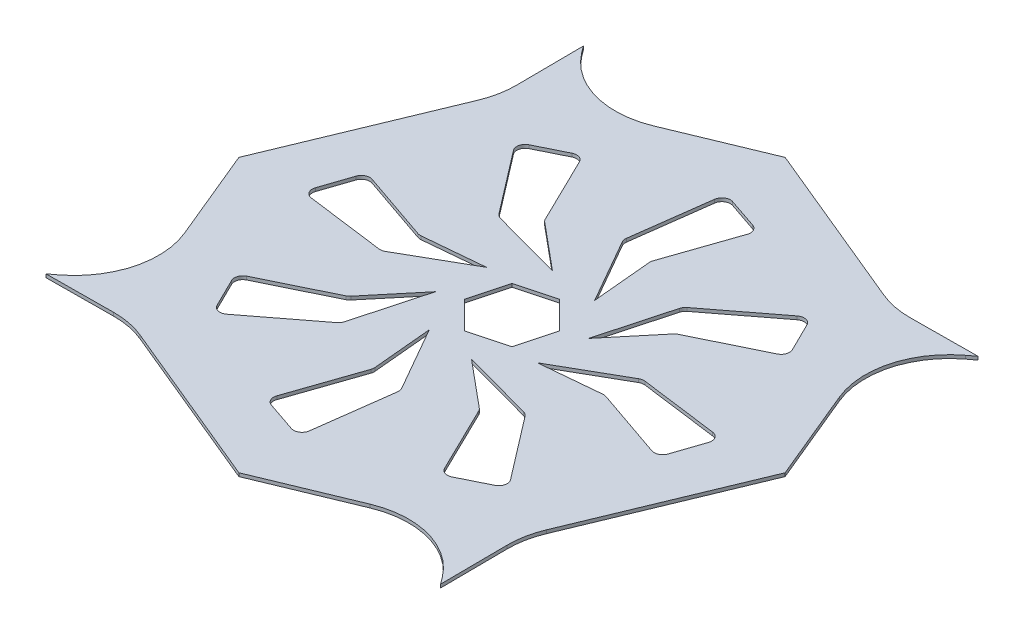
SolidWorks part; units mm, degrees
material "45"
ref_plane "Front Plane" through (0, 0, 0) normal (0, 0, 1) x (1, 0, 0)
ref_plane "Top Plane" through (0, 0, 0) normal (0, 1, 0) x (1, 0, 0)
ref_plane "Right Plane" through (0, 0, 0) normal (1, 0, 0) x (0, 0, -1)
sketch "Sketch1" plane through (0, 0, 0) normal (0, 1, 0) x (1, 0, 0)
  line L1 (114.805, -114.805) -> (162.3588, 0)
  line L2 (162.3588, 0) -> (114.805, 114.805)
  line L3 (114.805, 114.805) -> (0, 162.3588)
  line L4 (0, 162.3588) -> (-114.805, 114.805)
  line L5 (-114.805, 114.805) -> (-162.3588, 0)
  line L6 (-162.3588, 0) -> (-114.805, -114.805)
  line L7 (-114.805, -114.805) -> (0, -162.3588)
  line L8 (0, -162.3588) -> (114.805, -114.805)
  circle A0 centre (0, 0) radius 150 construction
  dimension "D1" = 300
extrude "Boss-Extrude1" add sketch "Sketch1" along normal blind 2
sketch "Sketch2" plane through (0, 2, 0) normal (0, 1, 0) x (1, 0, 0)
  line L0 (0, 0) -> (46.3685, 0) construction
  line L1 (22.3071, 5.9772) -> (5.9772, 22.3071)
  line L2 (5.9772, 22.3071) -> (-16.3299, 16.3299)
  line L3 (-16.3299, 16.3299) -> (-22.3071, -5.9772)
  line L4 (-22.3071, -5.9772) -> (-5.9772, -22.3071)
  line L5 (-5.9772, -22.3071) -> (16.3299, -16.3299)
  line L6 (16.3299, -16.3299) -> (22.3071, 5.9772)
  line L7 (0, 0) -> (16.3299, -16.3299) construction
  circle A0 centre (0, 0) radius 20 construction
  dimension "D1" = 40
  dimension "D2" = 45
extrude "Cut-Extrude1" cut sketch "Sketch2" against normal blind 10
sketch "Sketch3" plane through (0, 2, 0) normal (0, 1, 0) x (1, 0, 0)
  line L0 (7.1807, 123.975) -> (25.2073, 117.8588)
  line L1 (28.3287, 111.4971) -> (13.9987, 69.8505)
  line L2 (13.7476, 67.7664) -> (17.0204, 32.1308)
  line L3 (17.0204, 32.1308) -> (-4.8848, 70.4296)
  line L4 (-5.5015, 73.5667) -> (0.6173, 119.8948)
  line L5 (92.7411, 82.586) -> (101.163, 65.5145)
  line L6 (98.8718, 58.8089) -> (59.2903, 39.4932)
  line L7 (57.6391, 38.197) -> (34.7552, 10.6847)
  line L8 (34.7552, 10.6847) -> (46.3472, 53.2553)
  line L9 (48.1294, 55.9097) -> (85.2149, 84.3419)
  line L10 (123.975, -7.1807) -> (117.8588, -25.2073)
  line L11 (111.4971, -28.3287) -> (69.8505, -13.9987)
  line L12 (67.7664, -13.7476) -> (32.1308, -17.0204)
  line L13 (32.1308, -17.0204) -> (70.4296, 4.8848)
  line L14 (73.5667, 5.5015) -> (119.8948, -0.6173)
  line L15 (82.586, -92.7411) -> (65.5145, -101.163)
  line L16 (58.8089, -98.8718) -> (39.4932, -59.2903)
  line L17 (38.197, -57.6391) -> (10.6847, -34.7552)
  line L18 (10.6847, -34.7552) -> (53.2553, -46.3472)
  line L19 (55.9097, -48.1294) -> (84.3419, -85.2149)
  line L20 (-7.1807, -123.975) -> (-25.2073, -117.8588)
  line L21 (-28.3287, -111.4971) -> (-13.9987, -69.8505)
  line L22 (-13.7476, -67.7664) -> (-17.0204, -32.1308)
  line L23 (-17.0204, -32.1308) -> (4.8848, -70.4296)
  line L24 (5.5015, -73.5667) -> (-0.6173, -119.8948)
  line L25 (-92.7411, -82.586) -> (-101.163, -65.5145)
  line L26 (-98.8718, -58.8089) -> (-59.2903, -39.4932)
  line L27 (-57.6391, -38.197) -> (-34.7552, -10.6847)
  line L28 (-34.7552, -10.6847) -> (-46.3472, -53.2553)
  line L29 (-48.1294, -55.9097) -> (-85.2149, -84.3419)
  line L30 (-123.975, 7.1807) -> (-117.8588, 25.2073)
  line L31 (-111.4971, 28.3287) -> (-69.8505, 13.9987)
  line L32 (-67.7664, 13.7476) -> (-32.1308, 17.0204)
  line L33 (-32.1308, 17.0204) -> (-70.4296, -4.8848)
  line L34 (-73.5667, -5.5015) -> (-119.8948, 0.6173)
  line L35 (-82.586, 92.7411) -> (-65.5145, 101.163)
  line L36 (-58.8089, 98.8718) -> (-39.4932, 59.2903)
  line L37 (-38.197, 57.6391) -> (-10.6847, 34.7552)
  line L38 (-10.6847, 34.7552) -> (-53.2553, 46.3472)
  line L39 (-55.9097, 48.1294) -> (-84.3419, 85.2149)
  arc A0 (13.9987, 69.8505) -> (13.7476, 67.7664) centre (18.7267, 68.2237) ccw
  arc A1 (-4.8848, 70.4296) -> (-5.5015, 73.5667) centre (-0.5445, 72.912) cw
  arc A2 (0.6173, 119.8948) -> (7.1807, 123.975) centre (5.5743, 119.2401) cw
  arc A3 (28.3287, 111.4971) -> (25.2073, 117.8588) centre (23.6008, 113.1239) ccw
  circle A4 centre (0, 0) radius 14.7187 construction
  arc A5 (59.2903, 39.4932) -> (57.6391, 38.197) centre (61.4832, 34.9997) ccw
  arc A6 (46.3472, 53.2553) -> (48.1294, 55.9097) centre (51.1715, 51.9416) cw
  arc A7 (85.2149, 84.3419) -> (92.7411, 82.586) centre (88.2571, 80.3739) cw
  arc A8 (98.8718, 58.8089) -> (101.163, 65.5145) centre (96.679, 63.3024) ccw
  arc A9 (69.8505, -13.9987) -> (67.7664, -13.7476) centre (68.2237, -18.7267) ccw
  arc A10 (70.4296, 4.8848) -> (73.5667, 5.5015) centre (72.912, 0.5445) cw
  arc A11 (119.8948, -0.6173) -> (123.975, -7.1807) centre (119.2401, -5.5743) cw
  arc A12 (111.4971, -28.3287) -> (117.8588, -25.2073) centre (113.1239, -23.6008) ccw
  arc A13 (39.4932, -59.2903) -> (38.197, -57.6391) centre (34.9997, -61.4832) ccw
  arc A14 (53.2553, -46.3472) -> (55.9097, -48.1294) centre (51.9416, -51.1715) cw
  arc A15 (84.3419, -85.2149) -> (82.586, -92.7411) centre (80.3739, -88.2571) cw
  arc A16 (58.8089, -98.8718) -> (65.5145, -101.163) centre (63.3024, -96.679) ccw
  arc A17 (-13.9987, -69.8505) -> (-13.7476, -67.7664) centre (-18.7267, -68.2237) ccw
  arc A18 (4.8848, -70.4296) -> (5.5015, -73.5667) centre (0.5445, -72.912) cw
  arc A19 (-0.6173, -119.8948) -> (-7.1807, -123.975) centre (-5.5743, -119.2401) cw
  arc A20 (-28.3287, -111.4971) -> (-25.2073, -117.8588) centre (-23.6008, -113.1239) ccw
  arc A21 (-59.2903, -39.4932) -> (-57.6391, -38.197) centre (-61.4832, -34.9997) ccw
  arc A22 (-46.3472, -53.2553) -> (-48.1294, -55.9097) centre (-51.1715, -51.9416) cw
  arc A23 (-85.2149, -84.3419) -> (-92.7411, -82.586) centre (-88.2571, -80.3739) cw
  arc A24 (-98.8718, -58.8089) -> (-101.163, -65.5145) centre (-96.679, -63.3024) ccw
  arc A25 (-69.8505, 13.9987) -> (-67.7664, 13.7476) centre (-68.2237, 18.7267) ccw
  arc A26 (-70.4296, -4.8848) -> (-73.5667, -5.5015) centre (-72.912, -0.5445) cw
  arc A27 (-119.8948, 0.6173) -> (-123.975, 7.1807) centre (-119.2401, 5.5743) cw
  arc A28 (-111.4971, 28.3287) -> (-117.8588, 25.2073) centre (-113.1239, 23.6008) ccw
  arc A29 (-39.4932, 59.2903) -> (-38.197, 57.6391) centre (-34.9997, 61.4832) ccw
  arc A30 (-53.2553, 46.3472) -> (-55.9097, 48.1294) centre (-51.9416, 51.1715) cw
  arc A31 (-84.3419, 85.2149) -> (-82.586, 92.7411) centre (-80.3739, 88.2571) cw
  arc A32 (-58.8089, 98.8718) -> (-65.5145, 101.163) centre (-63.3024, 96.679) ccw
  point P110 (0, 0)
  dimension "D1" = 5
  dimension "D2" = 8
extrude "Cut-Extrude2" cut sketch "Sketch3" against normal blind 10
sketch "Sketch6" plane through (0, 2, 0) normal (0, 1, 0) x (1, 0, 0)
  line L0 (0, 0) -> (-114.805, 114.805) construction
  line L1 (-116.9103, 109.7225) -> (-117.2961, 159.7225)
  line L2 (-114.805, 114.805) -> (-162.3588, 0) construction
  line L3 (-117.2961, 159.7225) -> (-90.8359, 124.7334)
  line L4 (0, 162.3588) -> (-114.805, 114.805) construction
  line L5 (-90.8359, 124.7334) -> (-114.805, 114.805)
  line L6 (-114.805, 114.805) -> (-116.9103, 109.7225)
  line L7 (109.7225, 116.9103) -> (159.7225, 117.2961)
  line L8 (159.7225, 117.2961) -> (124.7334, 90.8359)
  line L9 (124.7334, 90.8359) -> (114.805, 114.805)
  line L10 (114.805, 114.805) -> (109.7225, 116.9103)
  line L11 (0, 0) -> (114.805, 114.805) construction
  line L12 (116.9103, -109.7225) -> (117.2961, -159.7225)
  line L13 (117.2961, -159.7225) -> (90.8359, -124.7334)
  line L14 (90.8359, -124.7334) -> (114.805, -114.805)
  line L15 (114.805, -114.805) -> (116.9103, -109.7225)
  line L16 (0, 0) -> (114.805, -114.805) construction
  line L17 (-109.7225, -116.9103) -> (-159.7225, -117.2961)
  line L18 (-159.7225, -117.2961) -> (-124.7334, -90.8359)
  line L19 (-124.7334, -90.8359) -> (-114.805, -114.805)
  line L20 (-114.805, -114.805) -> (-109.7225, -116.9103)
  line L21 (0, 0) -> (-114.805, -114.805) construction
  circle A0 centre (0, 0) radius 96.6837 construction
  point P27 (0, 0)
  dimension "D1" = 4
  dimension "D2" = 50
  dimension "D3" = 30
extrude "Boss-Extrude2" add sketch "Sketch6" against normal blind 2
fillet "Fillet1" radius 50 8 edges at (-116.9103, 1, -109.7225) (-90.8359, 1, -124.7334) (-124.7334, 1, 90.8359) (-109.7225, 1, 116.9103) (90.8359, 1, 124.7334) (116.9103, 1, 109.7225) (109.7225, 1, -116.9103) (124.7334, 1, -90.8359)
